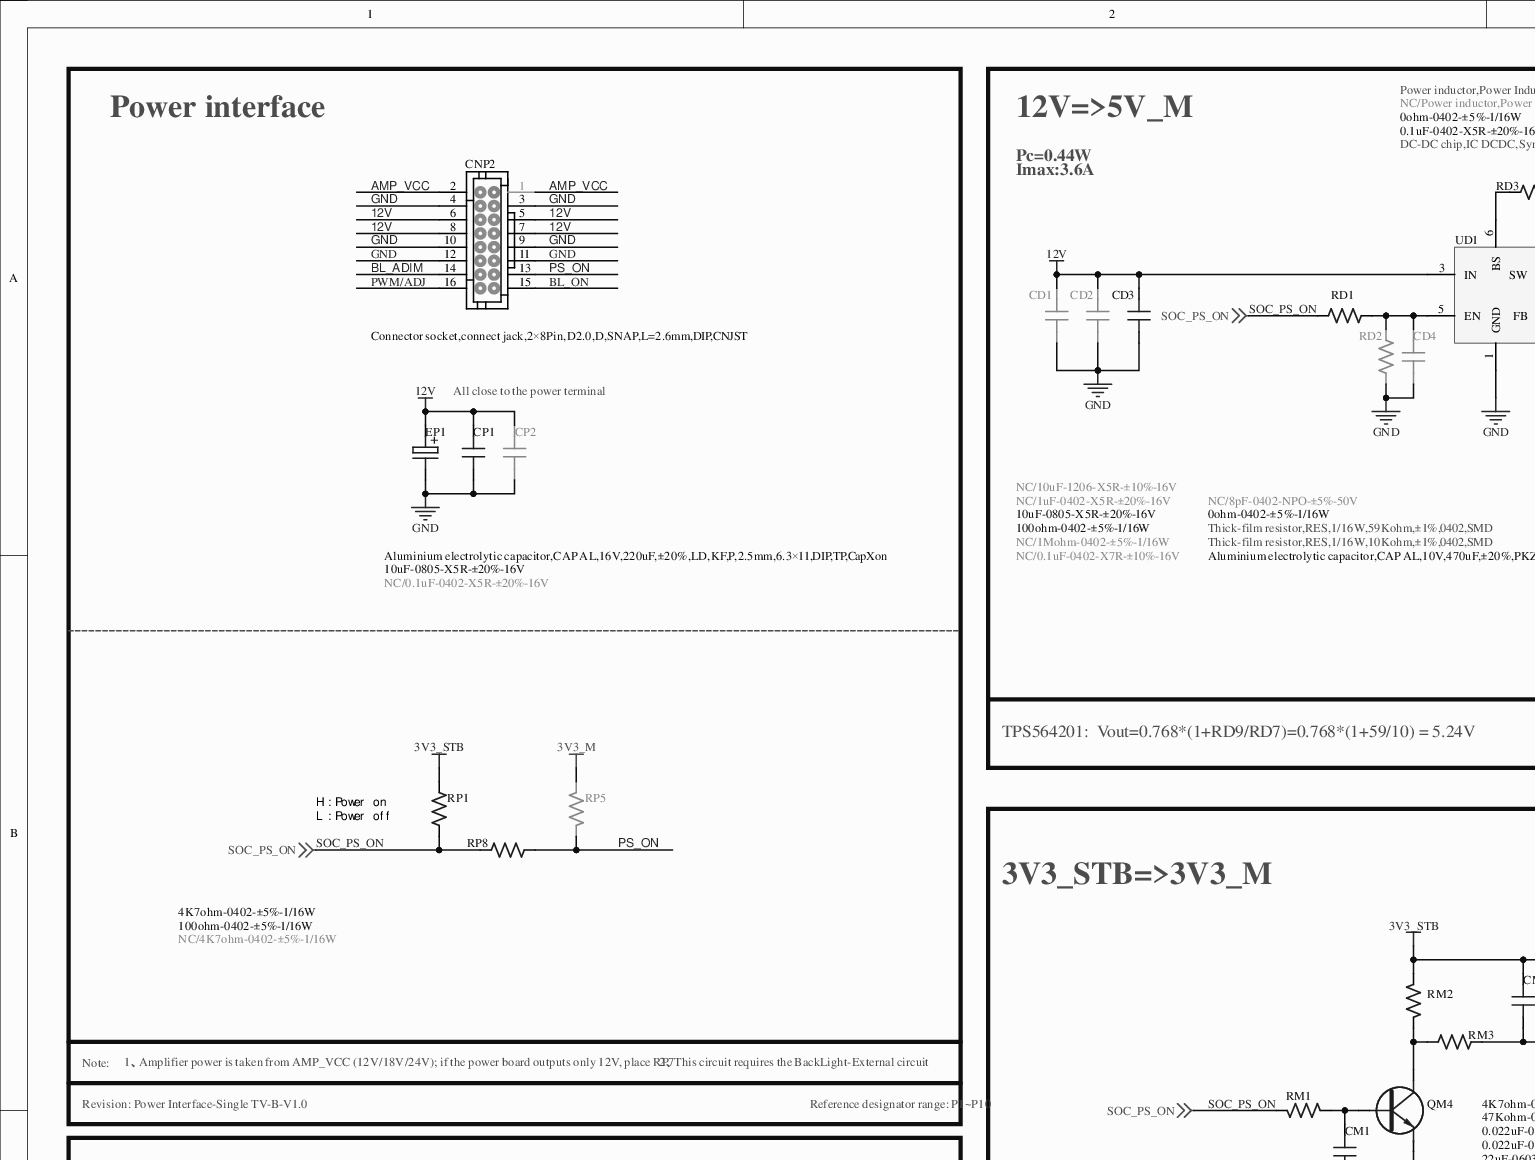
[diagram p0: MISC86290-6.SchDoc, top left]
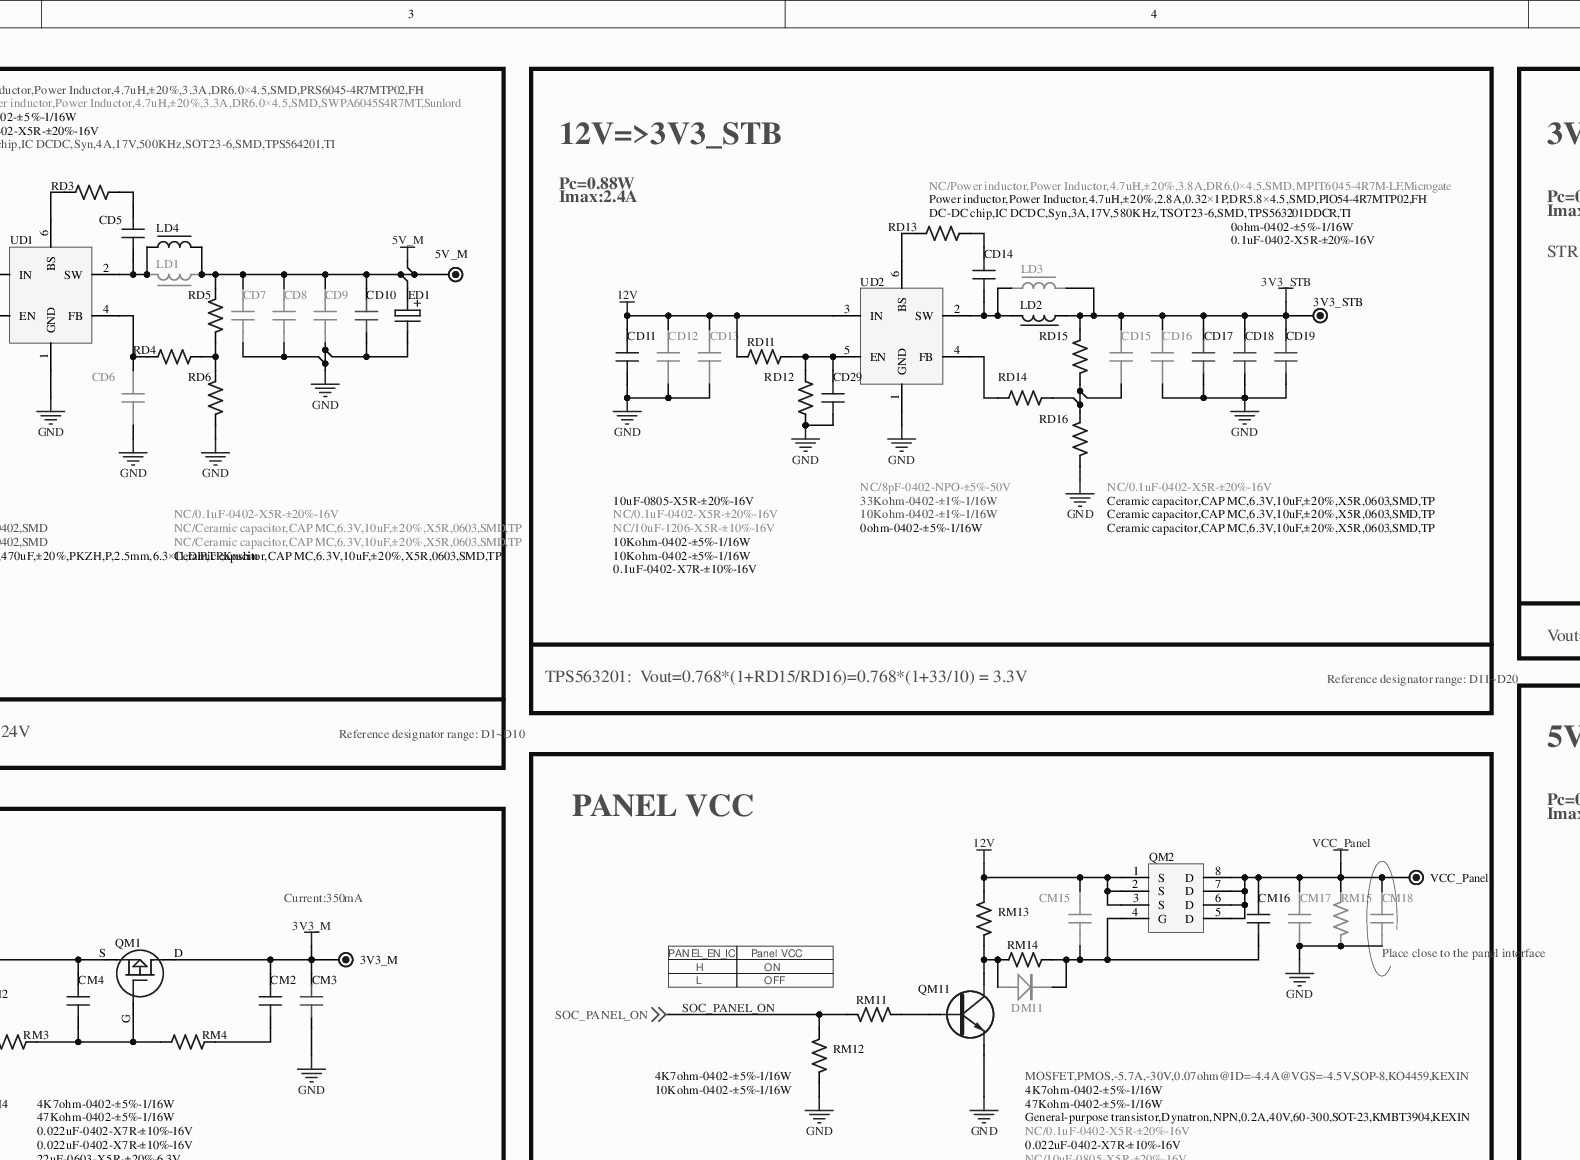
[diagram p1: MISC86290-6.SchDoc, top middle]
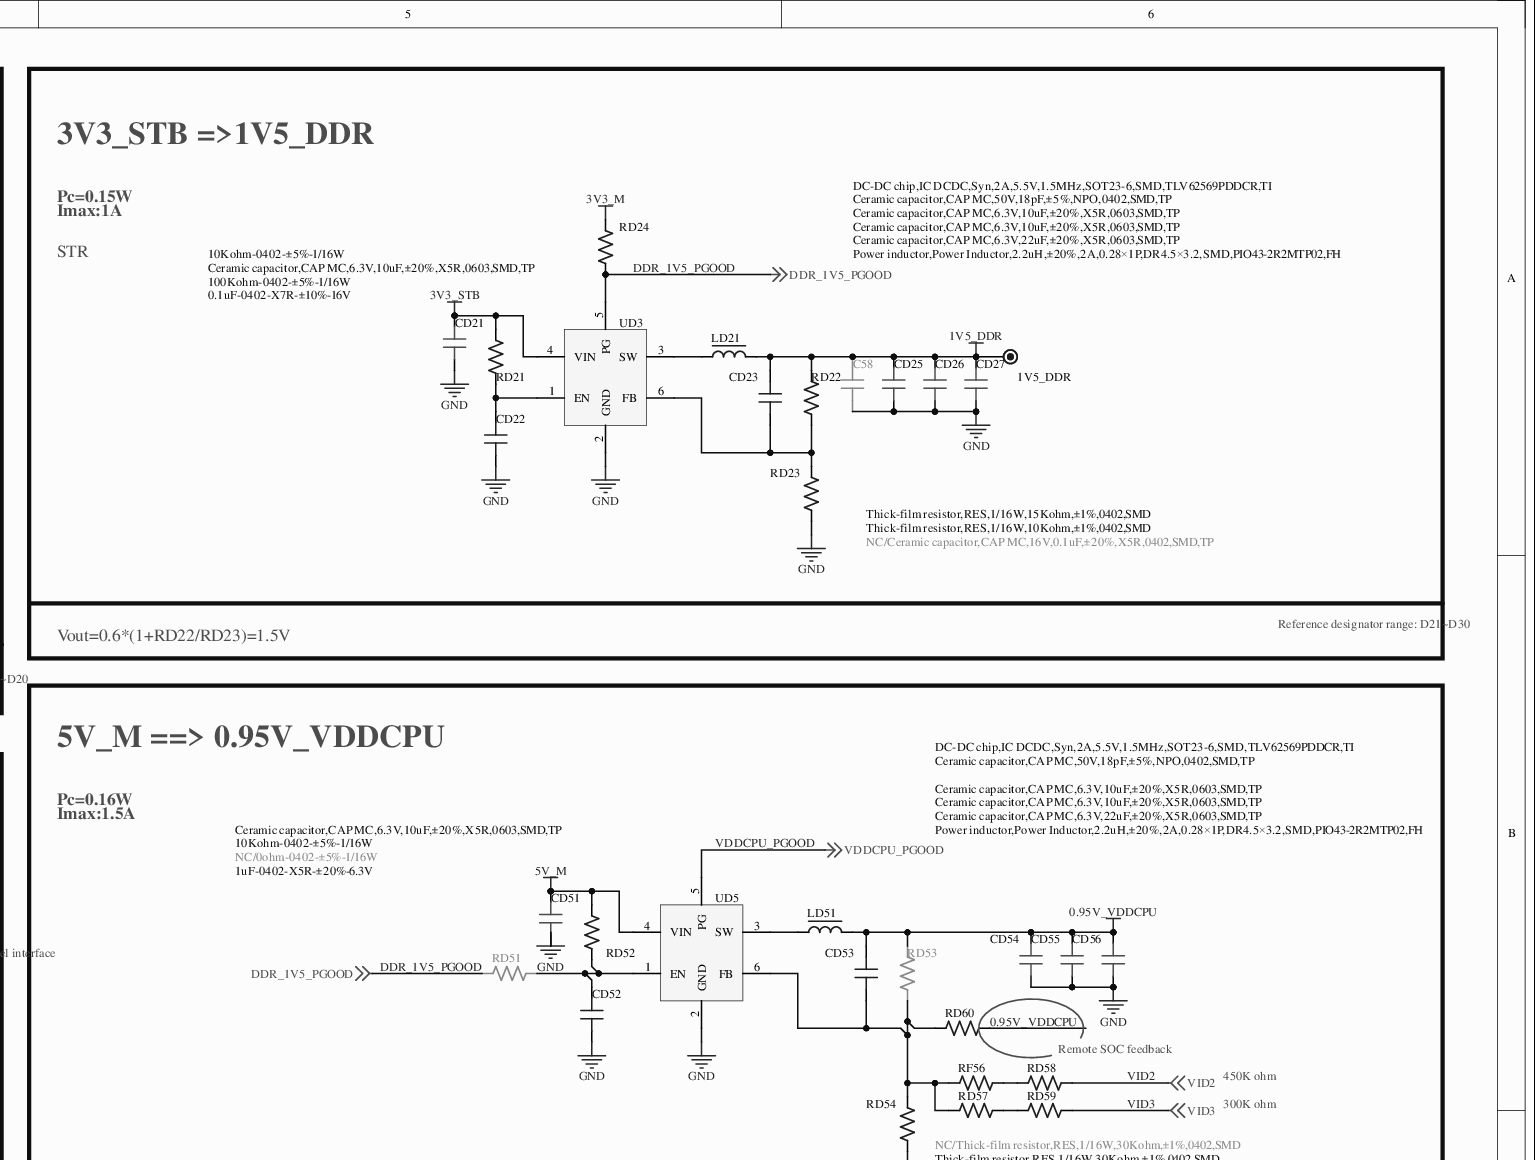
[diagram p2: MISC86290-6.SchDoc, top right]
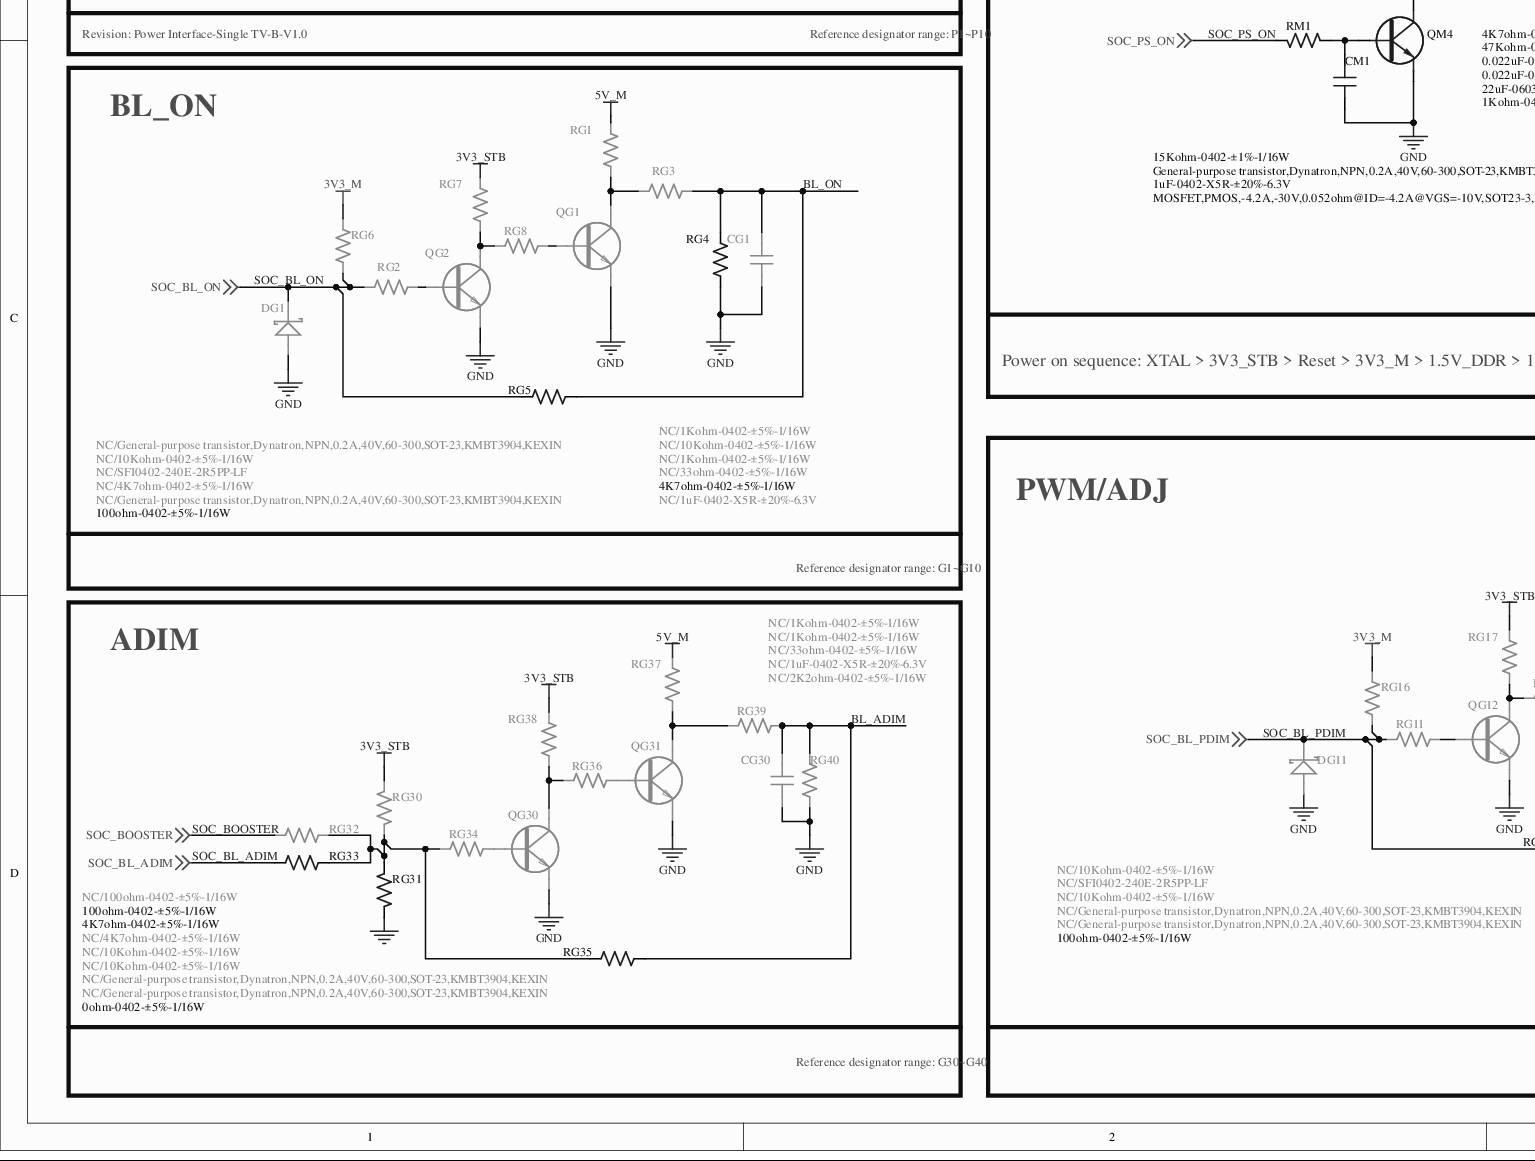
[diagram p3: MISC86290-6.SchDoc, bottom left]
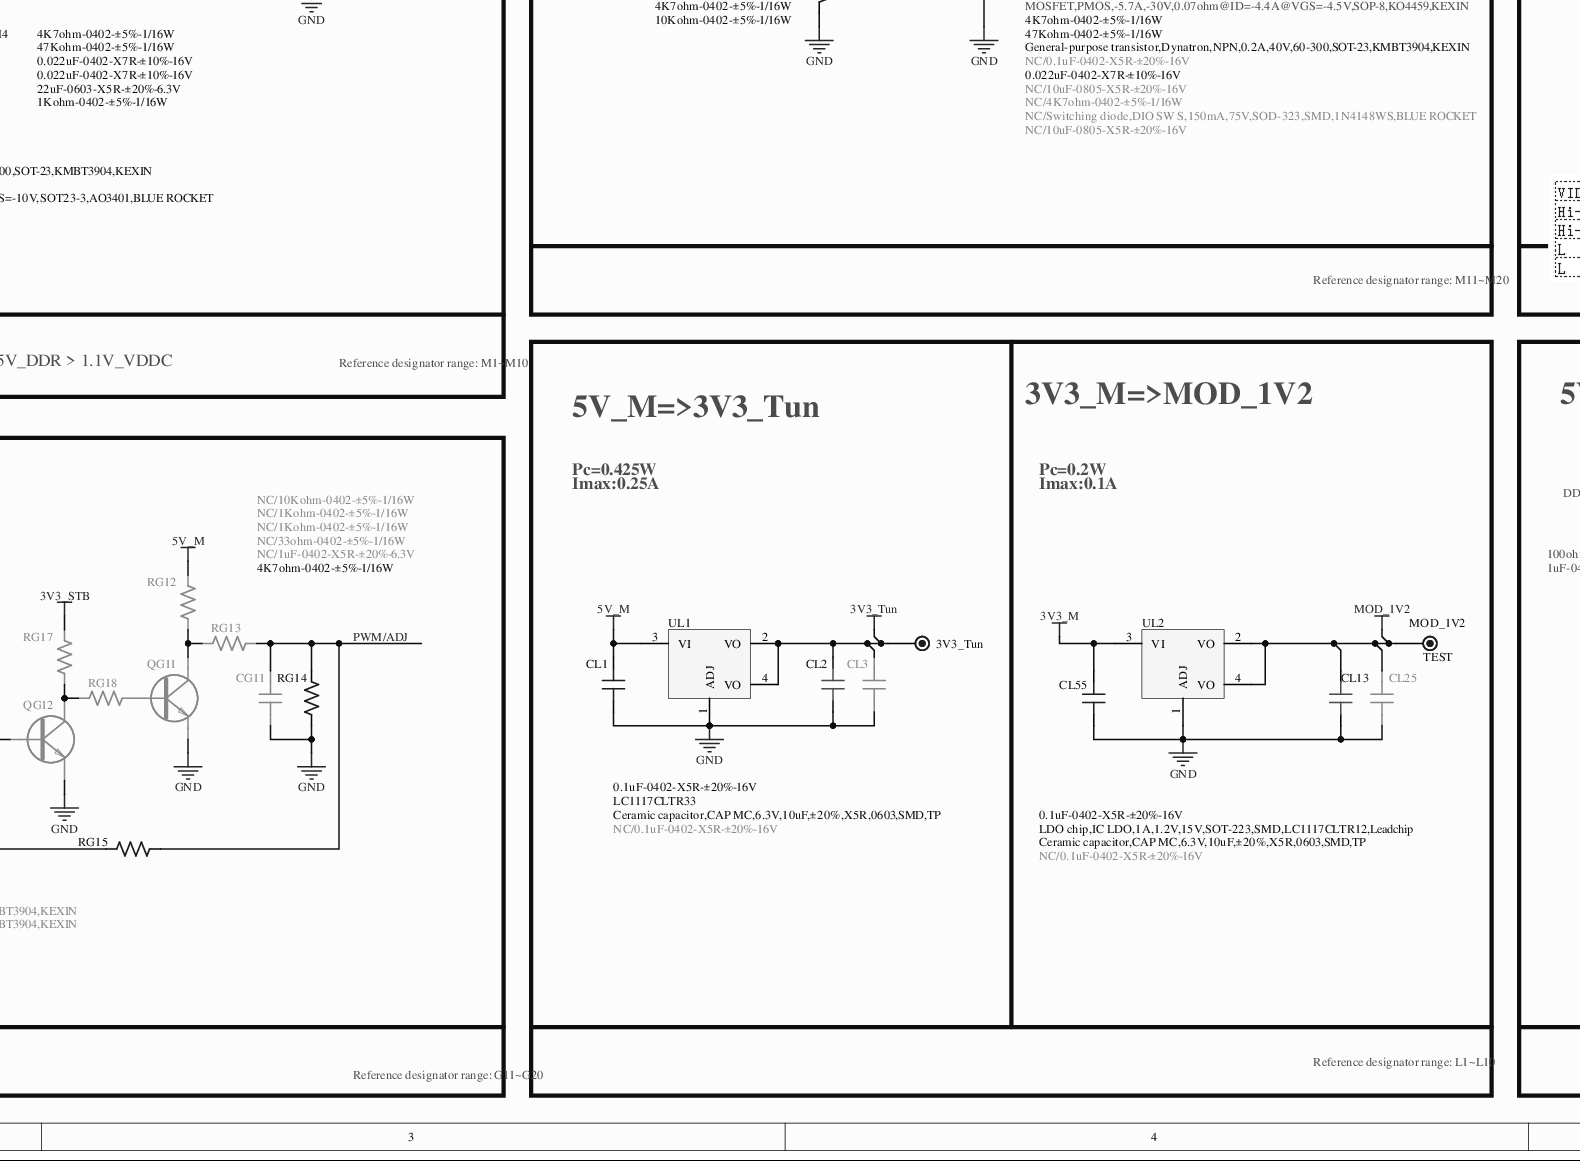
[diagram p4: MISC86290-6.SchDoc, bottom middle]
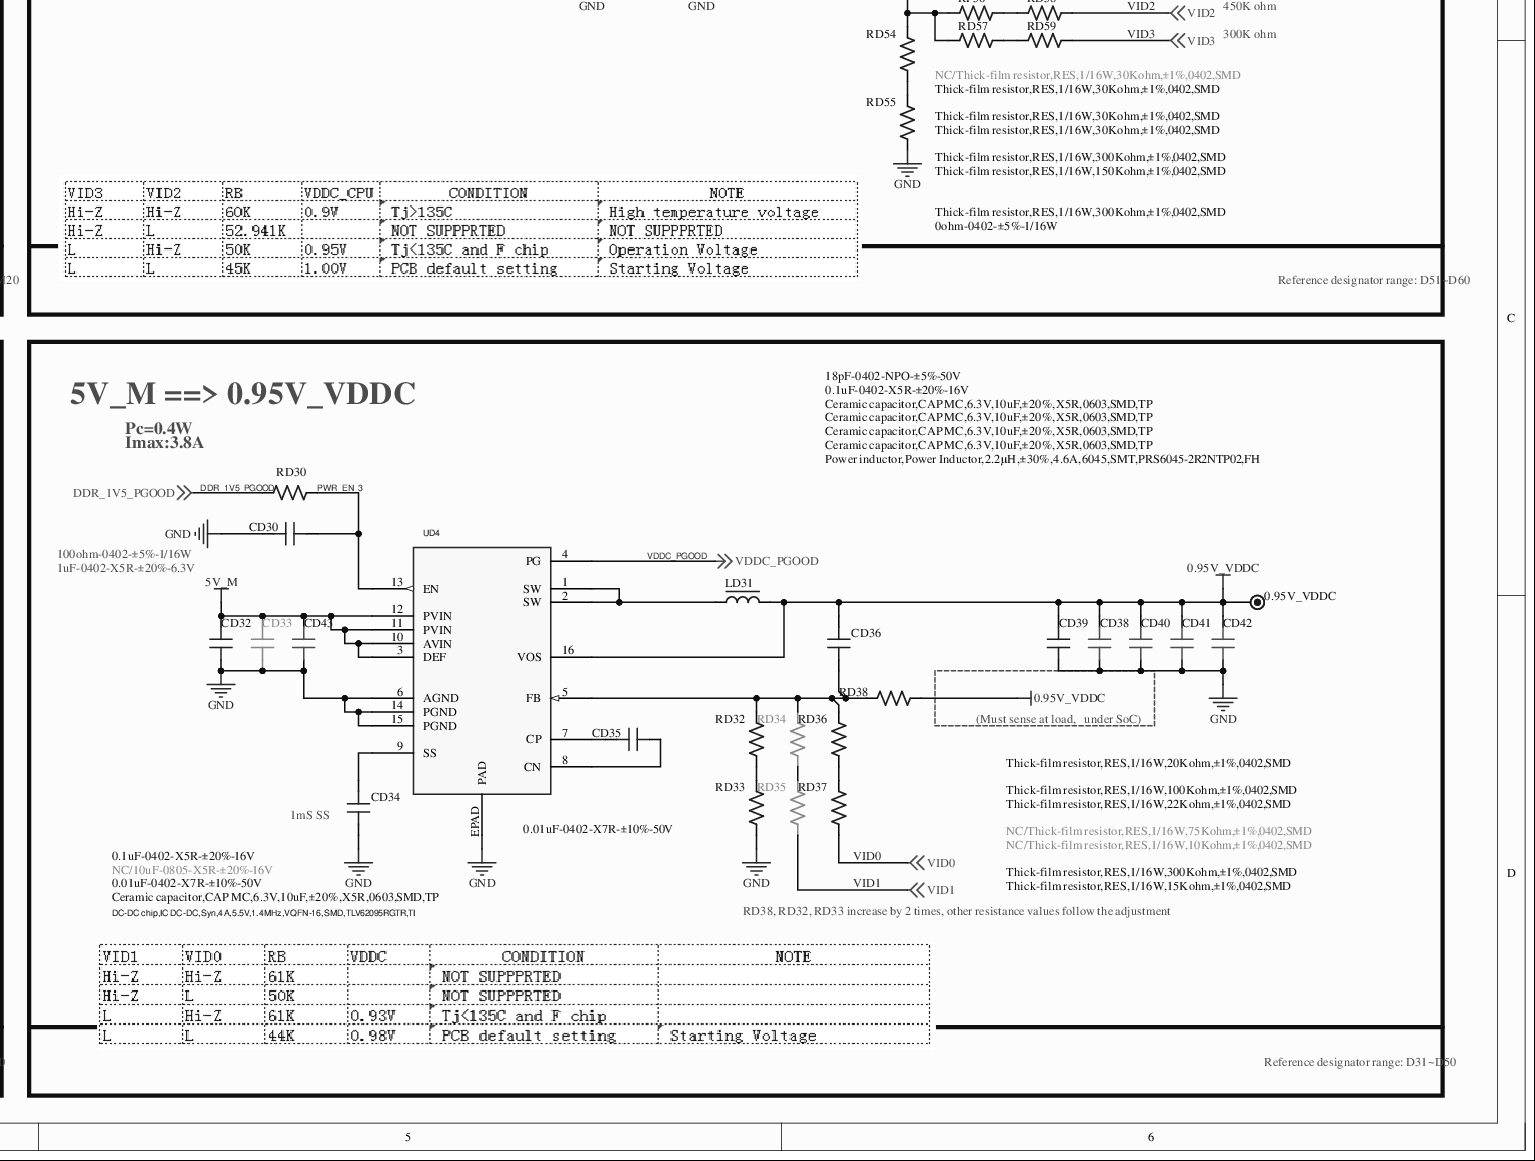
[diagram p5: MISC86290-6.SchDoc, bottom right]
# Altium project MISC86290.PrjPcb (part 4 of 13)

## Sheet MISC86290-6.SchDoc
size 825 x 411 mm